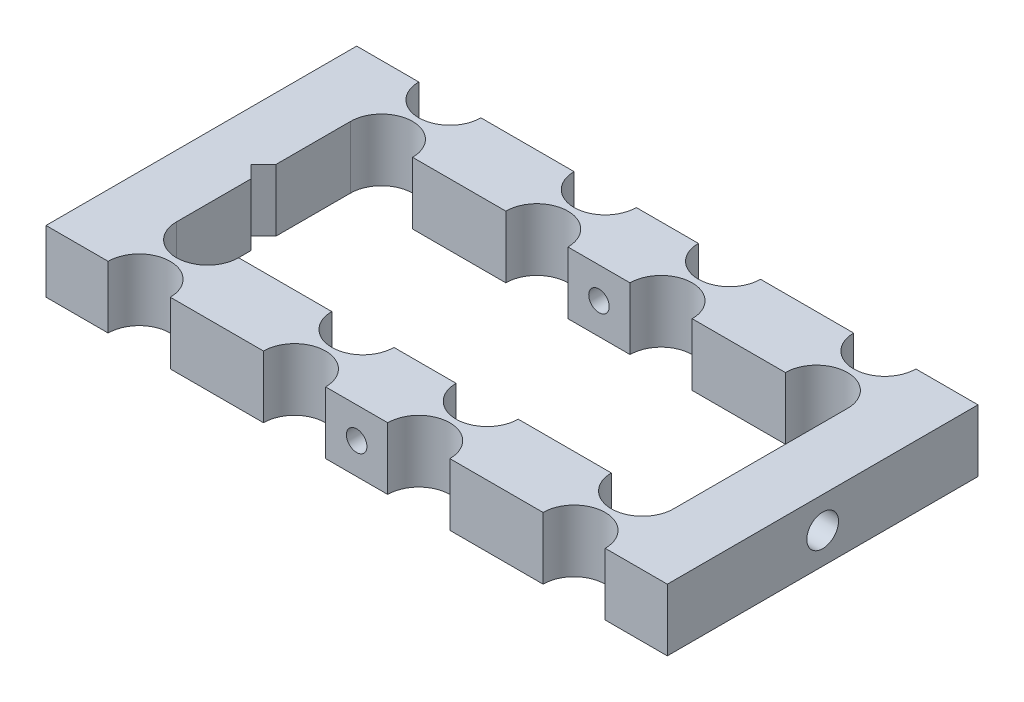
SolidWorks part; units mm, degrees
ref_plane "Front Plane" through (0, 0, 0) normal (0, 0, 1) x (1, 0, 0)
ref_plane "Top Plane" through (0, 0, 0) normal (0, 1, 0) x (1, 0, 0)
ref_plane "Right Plane" through (0, 0, 0) normal (1, 0, 0) x (0, 0, -1)
sketch "Sketch1" plane through (0, 0, 0) normal (0, 1, 0) x (1, 0, 0)
  line L0 (-1000, 0) -> (49000, 0) construction
  line L1 (-50, -25) -> (-40, -25)
  line L2 (-50, -25) -> (-50, 25)
  line L3 (-50, 25) -> (-40, 25)
  line L4 (50, -25) -> (50, 25)
  line L5 (0, -1000) -> (0, 49000) construction
  line L6 (-40, 14) -> (-40, 2)
  line L8 (-30, 14) -> (-15, 14)
  line L10 (-5, 14) -> (0, 14)
  line L11 (-30, -14) -> (-15, -14)
  line L12 (-5, -14) -> (5, -14)
  line L13 (-30, -25) -> (-15, -25)
  line L14 (-5, -25) -> (5, -25)
  line L15 (-30, 25) -> (-15, 25)
  line L16 (-5, 25) -> (5, 25)
  line L17 (-5, 14) -> (0, 14)
  line L18 (-30, 14) -> (-15, 14)
  line L19 (-5, -14) -> (5, -14)
  line L20 (-30, -14) -> (-15, -14)
  line L21 (30, -14) -> (15, -14)
  line L22 (30, -14) -> (15, -14)
  line L23 (30, 14) -> (15, 14)
  line L24 (30, 14) -> (15, 14)
  line L25 (40, 14) -> (40, -14)
  line L26 (15, 25) -> (30, 25)
  line L27 (40, 25) -> (50, 25)
  line L28 (15, -25) -> (30, -25)
  line L29 (40, -25) -> (50, -25)
  line L30 (0, 14) -> (5, 14)
  line L31 (-40, 2) -> (-42, 0)
  line L32 (-42, 0) -> (-40, -2)
  line L33 (-40, -2) -> (-40, -14)
  arc A0 (-40, 25) -> (-30, 25) centre (-35, 25) ccw
  arc A1 (-15, 25) -> (-5, 25) centre (-10, 25) ccw
  arc A2 (-30, 14) -> (-40, 14) centre (-35, 14) ccw
  arc A5 (-5, 14) -> (-15, 14) centre (-10, 14) ccw
  arc A6 (-5, -14) -> (-15, -14) centre (-10, -14) cw
  arc A7 (-30, -14) -> (-40, -14) centre (-35, -14) cw
  arc A8 (-15, -25) -> (-5, -25) centre (-10, -25) cw
  arc A9 (-40, -25) -> (-30, -25) centre (-35, -25) cw
  arc A10 (-40, 25) -> (-30, 25) centre (-35, 25) ccw
  arc A11 (-15, 25) -> (-5, 25) centre (-10, 25) ccw
  arc A12 (-30, 14) -> (-40, 14) centre (-35, 14) ccw
  arc A13 (-5, 14) -> (-15, 14) centre (-10, 14) ccw
  arc A14 (-5, -14) -> (-15, -14) centre (-10, -14) cw
  arc A15 (-30, -14) -> (-40, -14) centre (-35, -14) cw
  arc A16 (-15, -25) -> (-5, -25) centre (-10, -25) cw
  arc A17 (-40, -25) -> (-30, -25) centre (-35, -25) cw
  arc A18 (40, -25) -> (30, -25) centre (35, -25) ccw
  arc A19 (15, -25) -> (5, -25) centre (10, -25) ccw
  arc A20 (30, -14) -> (40, -14) centre (35, -14) ccw
  arc A21 (5, -14) -> (15, -14) centre (10, -14) ccw
  arc A22 (40, -25) -> (30, -25) centre (35, -25) ccw
  arc A23 (15, -25) -> (5, -25) centre (10, -25) ccw
  arc A24 (30, -14) -> (40, -14) centre (35, -14) ccw
  arc A25 (5, -14) -> (15, -14) centre (10, -14) ccw
  arc A26 (5, 14) -> (15, 14) centre (10, 14) cw
  arc A27 (30, 14) -> (40, 14) centre (35, 14) cw
  arc A28 (15, 25) -> (5, 25) centre (10, 25) cw
  arc A29 (40, 25) -> (30, 25) centre (35, 25) cw
  arc A30 (5, 14) -> (15, 14) centre (10, 14) cw
  arc A31 (30, 14) -> (40, 14) centre (35, 14) cw
  arc A32 (15, 25) -> (5, 25) centre (10, 25) cw
  arc A33 (40, 25) -> (30, 25) centre (35, 25) cw
  point P0 (0, 0)
  point P48 (0, -14)
  dimension "D3" = 15
  dimension "D4" = 25
  dimension "D5" = 10
  dimension "D6" = 25
  dimension "D8" = 10
  dimension "D10" = 11
  dimension "D1" = 100
  dimension "D2" = 50
  dimension "D7" = 15
  dimension "D9" = 11
  dimension "D11" = 2
  dimension "D12" = 2
  dimension "D13" = 2
extrude "Boss-Extrude1" add sketch "Sketch1" along normal blind 10 contours L27 A29 L26 A28 L16 A1 L15 A0 L3 L2 L1 A9 L13 A8 L14 A19 L28 A18 L29 L4 L23 A27 L25 A20 L21 A21 L12 A6 L11 A7 L6 A2 L8 A5 L10 L30 A26
hole_wizard "M4 Tapped Hole1" positions "Sketch2" profile "Sketch3" tap size "M4" standard "GB" end condition through all
sketch "Sketch2" plane through (0, 0, -25) normal (0, 0, -1) x (-1, 0, 0)
  line L0 (-5, 10) -> (-5, 0) construction
  line L1 (5, 10) -> (-5, 10) construction
  point P0 (0, 5)
  dimension "D1" = 5
  dimension "D2" = 5
sketch "Sketch3" plane through (0, 5, -25) normal (1, 0, 0) x (0, 1, 0)
  line L0 (0, 0) -> (0, 50)
  line L1 (0, 50) -> (1.65, 50)
  line L2 (1.65, 50) -> (1.65, 0)
  line L5 (1.65, 0) -> (0, 0)
  line L11 (0, -6.35) -> (0, 107.95) construction
  dimension "通孔螺纹孔钻头直径" = 3.3
  dimension "通孔螺纹孔钻头深度" = 50
cosmetic thread "Hole cosmetic thread1" parameters "D2"=4
sketch "Sketch4" plane through (-50, 0, 0) normal (-1, 0, 0) x (0, 0, 1)
  line L1 (25, 0) -> (-25, 0) construction
  circle A0 centre (0, 5) radius 2.55
  dimension "D1" = 5
  dimension "D2" = 5.1
extrude "Cut-Extrude1" cut sketch "Sketch4" against normal blind 84 from offset 30 offset against normal yes
scale "Scale factor1" scale about origin uniform scaling yes scale factor 0.7
